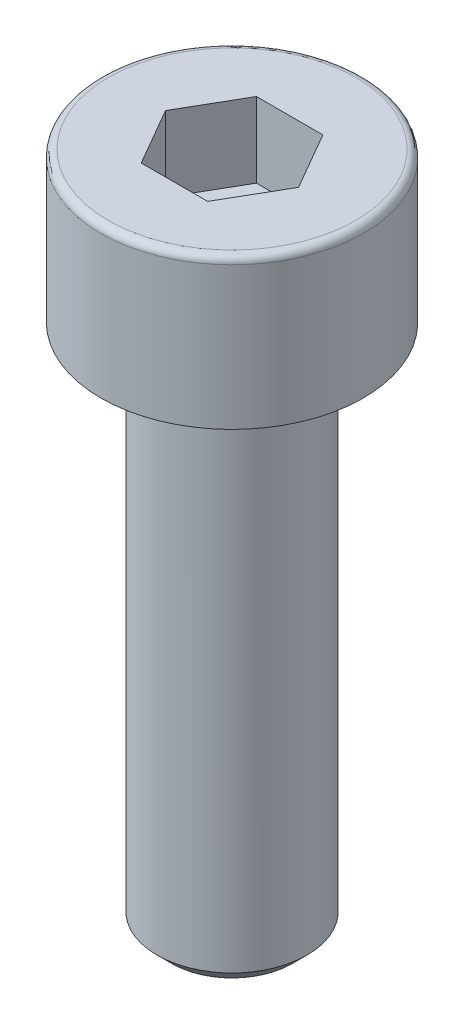
from build123d import *

# Parameters (mm, degrees)
SKETCH_1_R          = 3.5
EXTRUDE_1_DEPTH     = 4
CUT_EXTRUDE_1_DEPTH = 2
FILLET_1_R          = 0.2
SKETCH_5_R          = 2
EXTRUDE_2_DEPTH     = 14
CHAMFER_2_SIZE      = 0.39


with BuildPart() as part:
    # 草图1 → 凸台-拉伸1 (new body)
    with BuildSketch(Plane(origin=(0, 0, 0), x_dir=(1, 0, 0), z_dir=(0, 1, 0))):
        with Locations(Location((0, 0, 0), (0, 0, 270))):
            Circle(SKETCH_1_R)
    extrude(amount=EXTRUDE_1_DEPTH)

    # 草图2 → 切除-拉伸1 (cut)
    with BuildSketch(Plane(origin=(0, 4, 0), x_dir=(1, 0, 0), z_dir=(0, 1, 0))):
        Polygon((1.772465326, 0), (0.886232663, 1.535), (-0.886232663, 1.535), (-1.772465326, 0), (-0.886232663, -1.535), (0.886232663, -1.535), align=None)
    extrude(amount=-CUT_EXTRUDE_1_DEPTH, mode=Mode.SUBTRACT)

    # 圆角1
    fillet_1_edges = [part.edges().sort_by_distance(p)[0] for p in [
        (0, 4, -3.5),
    ]]
    fillet(fillet_1_edges, radius=FILLET_1_R)

    # 草图5 → 凸台-拉伸2 (add)
    with BuildSketch(Plane.XZ):
        with Locations(Location((0, 0, 0), (0, 0, 90))):
            Circle(SKETCH_5_R)
    extrude(amount=EXTRUDE_2_DEPTH)

    # 倒角2
    chamfer_2_edges = [part.edges().sort_by_distance(p)[0] for p in [
        (0, -14, -2),
    ]]
    chamfer(chamfer_2_edges, length=CHAMFER_2_SIZE)


solid = part.part
